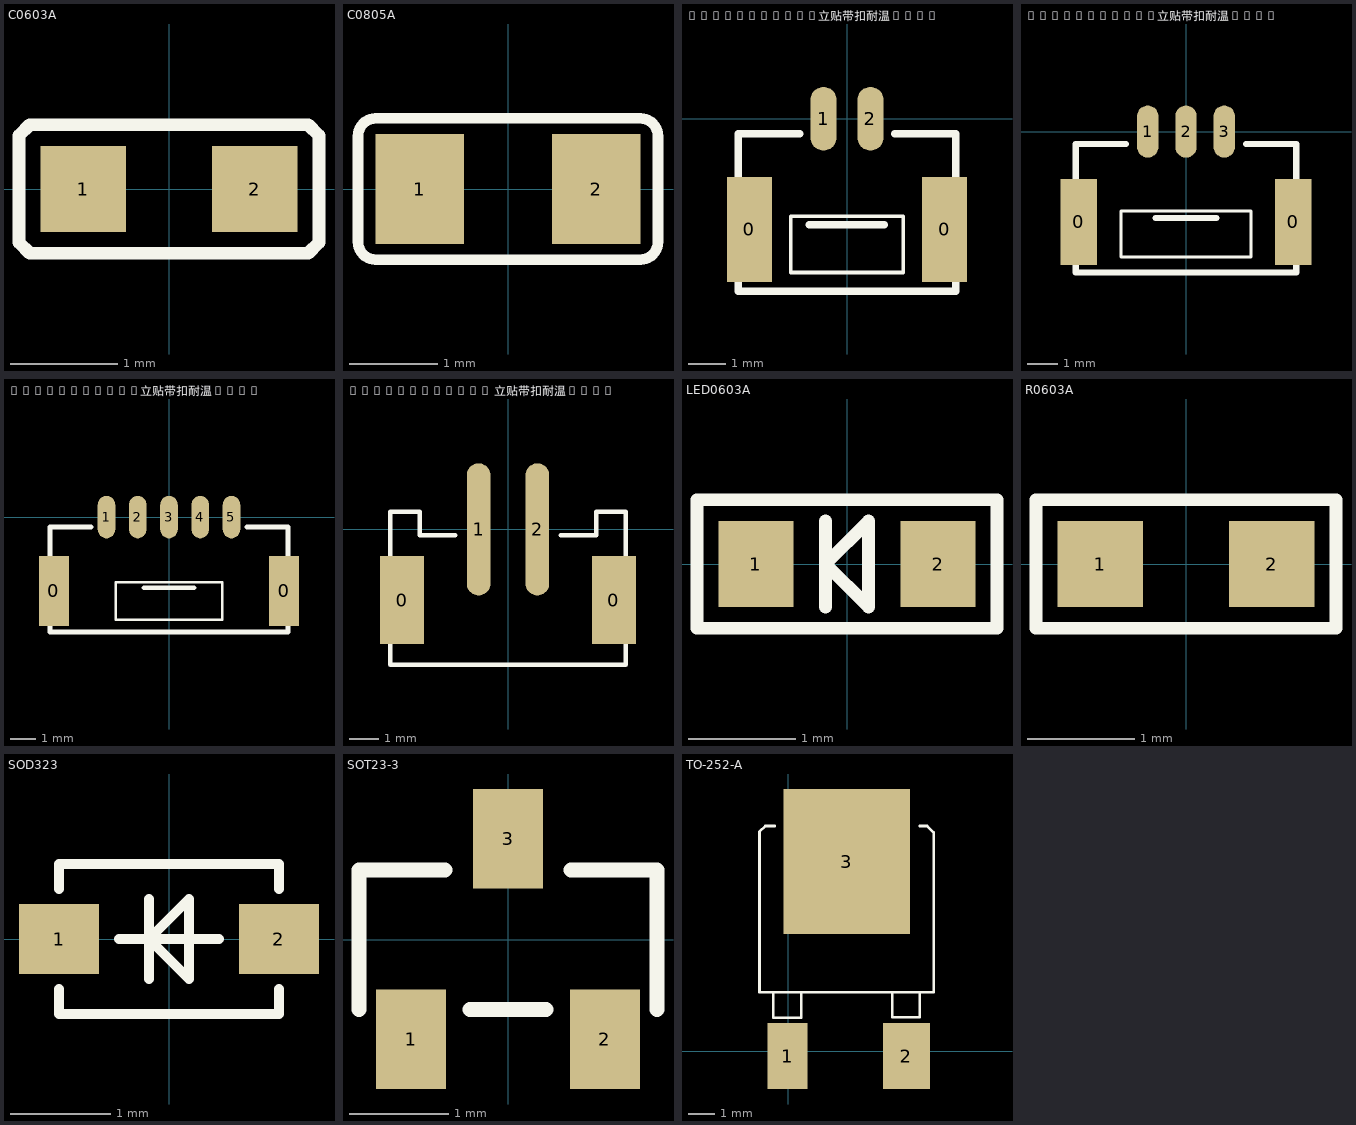
[diagram p0: the footprints below, top view; thin cyan lines are the x and y axes]
# Altium footprint library MISC88840.PcbLib: 11 footprints
Each footprint in its own frame and in the unit in brackets; x right, y up, seen from the top. Pads: shape width x height; smd on the part's side, far side on the other; paste and mask are expansions set on the pad; w line width, h text height; cw(c..) or ccw(c..) is an arc to the next point about the centre after c.

## C0603A [mm] "SMD capacitor"
pads (2):
  rect 0.8x0.8 smd mask+0.08: 1(-0.8,0) 2(0.8,0)
Top Overlay:
  lines w0.12: 0.551,-0.6 1.2,-0.6 ; -1.4,-0.5 -1.4,0.5 -1.3,0.6 1.3,0.6 1.4,0.5 1.4,-0.5 1.3,-0.6 -1.3,-0.6 -1.4,-0.5

## C0805A [mm] "SMD capacitor"
pads (2):
  rect 1x1.25 smd: 1(-1,0)
  rect 1x1.25 smd mask+0.102: 2(1,0)
Top Overlay:
  lines w0.12: -1.7,-0.6 ccw(c-1.5,-0.6) -1.5,-0.8 1.5,-0.8 ccw(c1.5,-0.6) 1.7,-0.6 1.7,0.6 ccw(c1.5,0.6) 1.5,0.8 -1.5,0.8 ccw(c-1.5,0.6) -1.7,0.6 -1.7,-0.6

## GH1.25-2PIN立贴带扣耐温260℃ [mm] "Vertical SMD with latch, heat resistant 260℃"
pads (4):
  rect 1.2x2.8 smd: 0(-2.6,-2.95) 0(2.6,-2.95)
  oval 0.7x1.7 smd: 1(-0.625,0) 2(0.625,0)
Top Overlay:
  lines w0.1: -1.5,-4.1 -1.5,-2.6 1.5,-2.6 1.5,-4.1 -1.5,-4.1
  lines w0.2: -2.9,-0.4 -2.9,-4.6 2.9,-4.6 2.9,-0.4 1.27,-0.4 ; -2.895,-0.4 -1.265,-0.4 ; -1,-2.825 1,-2.825

## GH1.25-3PIN立贴带扣耐温260℃ [mm] "Vertical SMD with latch, heat resistant 260℃"
pads (5):
  rect 1.2x2.8 smd: 0(-3.5,-2.95) 0(3.5,-2.95)
  oval 0.7x1.7 smd: 1(-1.25,0) 2(0,0) 3(1.25,0)
Top Overlay:
  lines w0.1: -2.125,-4.1 -2.125,-2.6 2.125,-2.6 2.125,-4.1 -2.125,-4.1
  lines w0.2: -3.6,-0.4 -3.6,-4.6 3.6,-4.6 3.6,-0.4 ; -3.595,-0.4 -1.965,-0.4 ; -1,-2.825 1,-2.825 ; 1.96,-0.4 3.59,-0.4

## GH1.25-5PIN立贴带扣耐温260℃ [mm] "Vertical SMD with latch, heat resistant 260℃"
pads (7):
  rect 1.2x2.8 smd: 0(-4.6,-2.95) 0(4.6,-2.95)
  oval 0.7x1.7 smd: 1(-2.5,0) 2(-1.25,0) 3(0,0) 4(1.25,0) 5(2.5,0)
Top Overlay:
  lines w0.1: -2.125,-4.1 -2.125,-2.6 2.125,-2.6 2.125,-4.1 -2.125,-4.1
  lines w0.2: -3.125,-0.4 -4.755,-0.4 -4.755,-4.6 4.755,-4.6 4.755,-0.4 ; -1,-2.825 1,-2.825 ; 3.12,-0.4 4.75,-0.4

## HY2.0WT-2A/P 立贴带扣耐温260℃ [mm] "Horizontal SMD connector"
pads (4):
  rect 1.5x3 smd: 0(-3.6,-2.4) 0(3.6,-2.4)
  oval 0.8x4.5 smd: 1(-1,0) 2(1,0)
Top Overlay:
  lines w0.15: -1.8,-0.2 -3,-0.2 -3,0.6 -4,0.6 -4,-4.6 4,-4.6 4,0.6 3,0.6 3,-0.2 1.8,-0.2

## LED0603A [mm] "SMD LED"
pads (2):
  rect 0.7x0.8 smd: 1(-0.85,0) 2(0.85,0)
Top Overlay:
  lines w0.12: -0.2,-0.4 -0.2,0.4 ; -1.4,-0.6 -1.4,0.6 1.4,0.6 1.4,-0.6 -1.4,-0.6 ; -0.2,0 0.2,0.4 0.2,-0.4 -0.2,0

## R0603A [mm] "SMD resistor"
height 0.5
pads (2):
  rect 0.8x0.8 smd mask+0.08: 1(-0.8,0) 2(0.8,0)
Top Overlay:
  lines w0.12: -1.4,-0.6 -1.4,0.6 1.4,0.6 1.4,-0.6 -1.4,-0.6

## SOD323 [mm] "SMD diode"
pads (2):
  rect 0.8x0.7 smd: 1(-1.1,0) 2(1.1,0)
Top Overlay:
  lines w0.1: -1.1,-0.5 -1.1,-0.75 1.1,-0.75 1.1,-0.5 ; -1.1,0.5 -1.1,0.75 1.1,0.75 1.1,0.5 ; -0.5,0 0.5,0 ; -0.2,-0.4 -0.2,0.4 ; -0.2,0 0.2,0.4 0.2,-0.4 -0.2,0

## SOT23-3 [mm] "SMD IC/MOS*"
pads (3):
  rect 0.7x1 smd: 1(-0.975,-1) 2(0.975,-1) 3(0,1.016)
Top Overlay:
  lines w0.15: -1.5,-0.7 -1.5,0.7 -0.635,0.7 ; -0.381,-0.7 0.381,-0.7 ; 0.635,0.7 1.5,0.7 1.5,-0.7

## TO-252-A [mm]
height 2.5
pads (3):
  rect 1.5x2.5 smd: 1(-0.026,-0.189)
  rect 1.8x2.5 smd: 2(4.484,-0.189)
  rect 4.8x5.5 smd: 3(2.214,7.181)
Top Overlay:
  lines w0.1: -0.561,2.231 -0.561,1.256 0.489,1.256 0.489,2.181 ; -0.511,8.531 -0.869,8.531 -1.086,8.314 -1.086,2.231 5.514,2.231 5.514,8.286 5.269,8.531 4.989,8.531 ; 3.939,2.231 3.939,1.281 4.989,1.281 4.989,2.231
3D body: height 2.5, standoff 0, extent -0.95,8.05 -0.95,8.15
3D body: height 0.5, standoff 0, extent -0.95,2.3 5.35,8.25
3D body: height 0.5, standoff 0, extent 1.6,1.3 2.65,2.55
3D body: height 0.5, standoff 0, extent 3.9,-0.35 4.95,2.15
3D body: height 0.5, standoff 0, extent -0.6,-0.25 0.45,2.25
3D body: height 0.5, standoff 0, extent -0.95,8.1 5.25,9.65